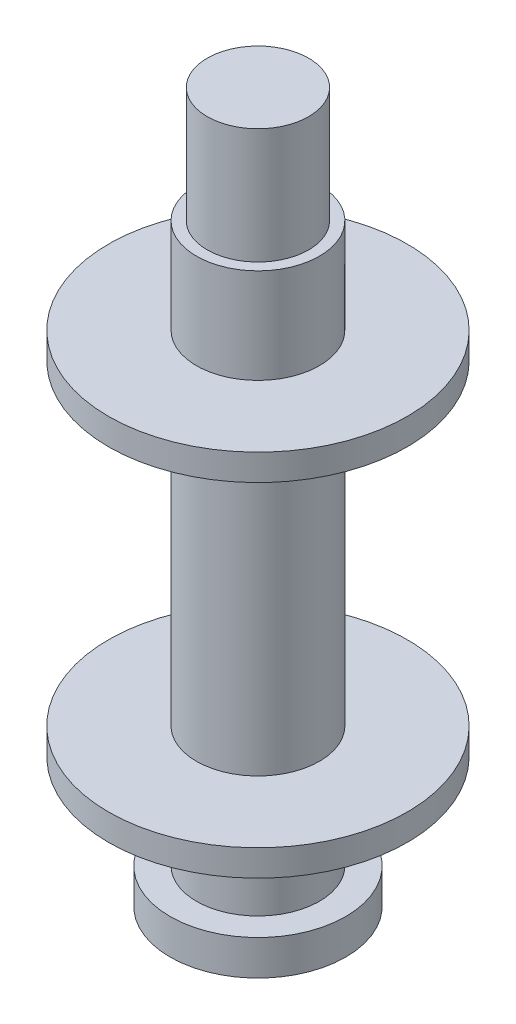
SolidWorks part; units mm, degrees
material "AISI 1045 钢，冷拔"
ref_plane "Front Plane" through (0, 0, 0) normal (0, 0, 1) x (1, 0, 0)
ref_plane "Top Plane" through (0, 0, 0) normal (0, 1, 0) x (1, 0, 0)
ref_plane "Right Plane" through (0, 0, 0) normal (1, 0, 0) x (0, 0, -1)
sketch "Sketch1" plane through (0, 0, 0) normal (0, 1, 0) x (1, 0, 0)
  circle A0 centre (0, 0) radius 5
extrude "Boss-Extrude1" add sketch "Sketch1" along normal blind 2
ref_plane "Plane1" through (0, 2, 0) normal (0, 1, 0) x (1, 0, 0)
sketch "Sketch2" plane through (0, 2, 0) normal (0, 1, 0) x (1, 0, 0)
  circle A0 centre (0, 0) radius 3.5
extrude "Boss-Extrude2" add sketch "Sketch2" along normal blind 5.4
ref_plane "Plane2" through (0, 7.4, 0) normal (0, 1, 0) x (1, 0, 0)
sketch "Sketch3" plane through (0, 7.4, 0) normal (0, 1, 0) x (1, 0, 0)
  circle A0 centre (0, 0) radius 8.5
extrude "Boss-Extrude3" add sketch "Sketch3" along normal blind 1.5
ref_plane "Plane3" through (0, 8.9, 0) normal (0, 1, 0) x (1, 0, 0)
sketch "Sketch4" plane through (0, 8.9, 0) normal (0, 1, 0) x (1, 0, 0)
  circle A0 centre (0, 0) radius 3.5
extrude "Boss-Extrude4" add sketch "Sketch4" along normal blind 18
ref_plane "Plane4" through (0, 26.9, 0) normal (0, 1, 0) x (1, 0, 0)
sketch "Sketch5" plane through (0, 26.9, 0) normal (0, 1, 0) x (1, 0, 0)
  circle A0 centre (0, 0) radius 8.5
extrude "Boss-Extrude5" add sketch "Sketch5" along normal blind 1.5
ref_plane "Plane5" through (0, 28.4, 0) normal (0, 1, 0) x (1, 0, 0)
sketch "Sketch6" plane through (0, 28.4, 0) normal (0, 1, 0) x (1, 0, 0)
  circle A0 centre (0, 0) radius 3.5
extrude "Boss-Extrude6" add sketch "Sketch6" along normal blind 5.4
ref_plane "Plane6" through (0, 33.8, 0) normal (0, 1, 0) x (1, 0, 0)
sketch "Sketch7" plane through (0, 33.8, 0) normal (0, 1, 0) x (1, 0, 0)
  circle A0 centre (0, 0) radius 2.885
extrude "Boss-Extrude7" add sketch "Sketch7" along normal blind 6.57
